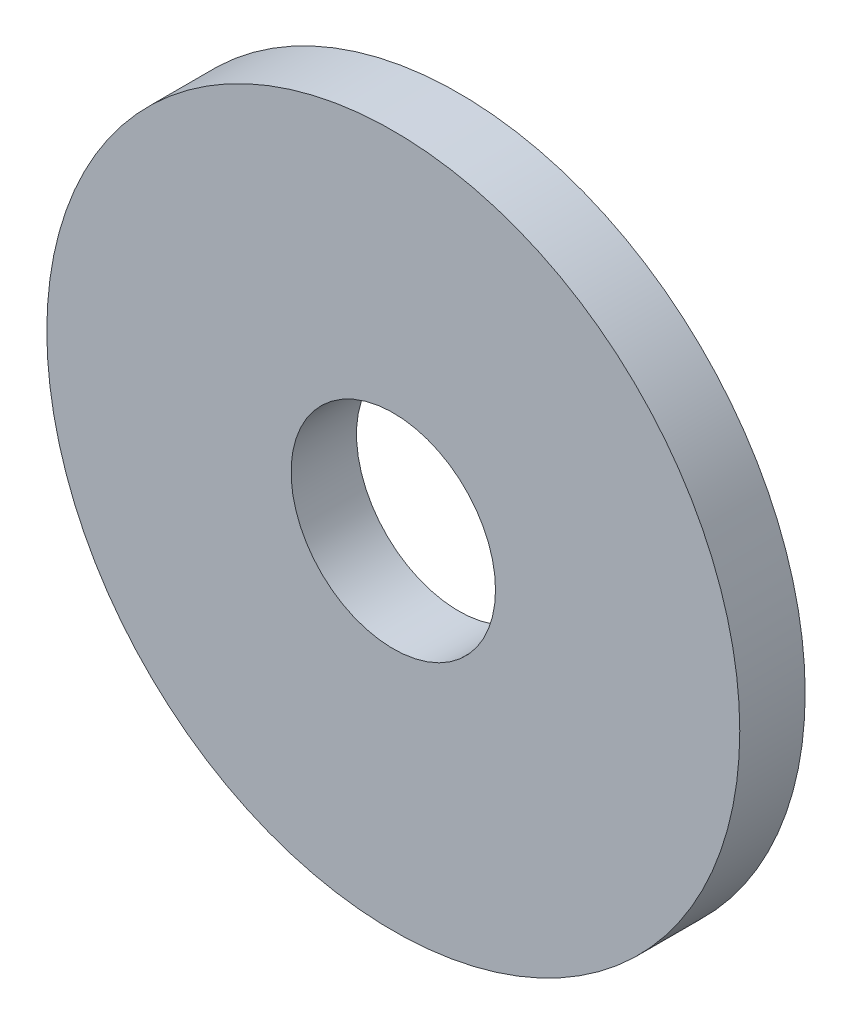
SolidWorks part; units mm, degrees
ref_plane "Front Plane" through (0, 0, 0) normal (0, 0, 1) x (1, 0, 0)
ref_plane "Top Plane" through (0, 0, 0) normal (0, 1, 0) x (1, 0, 0)
ref_plane "Right Plane" through (0, 0, 0) normal (1, 0, 0) x (0, 0, -1)
sketch "Sketch1" plane through (0, 0, 0) normal (0, 0, 1) x (1, 0, 0)
  circle A0 centre (0, 0) radius 84.75
  circle A1 centre (0, 0) radius 25
  dimension "D1" = 169.5
  dimension "D2" = 50
extrude "Boss-Extrude1" add sketch "Sketch1" along normal blind 16 contours A0 | A1
